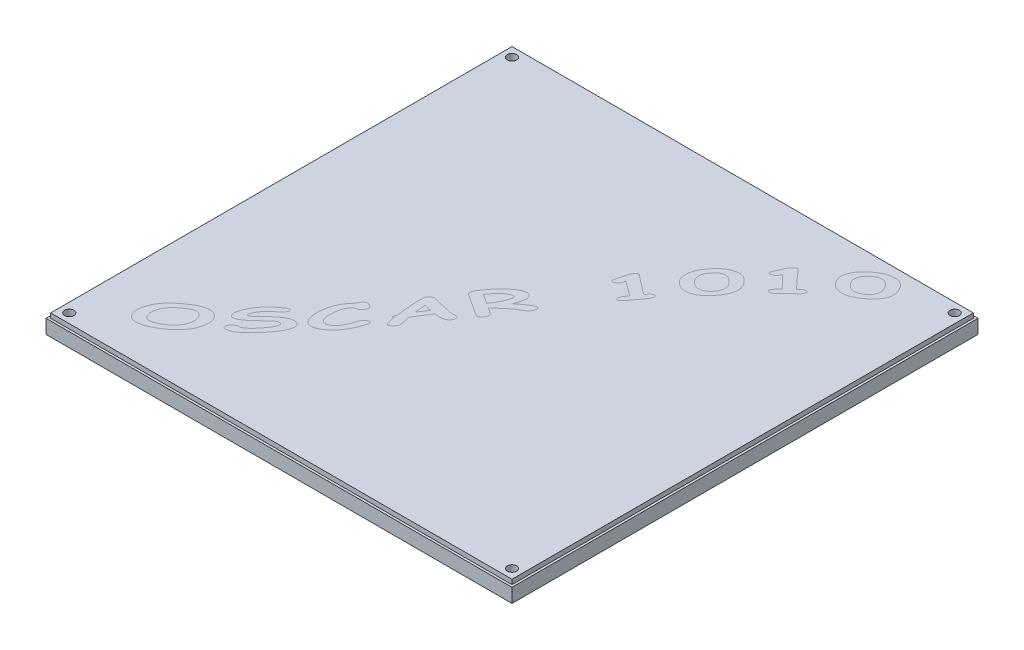
SolidWorks part; units mm, degrees
material "Brass"
ref_plane "Front Plane" through (0, 0, 0) normal (0, 0, 1) x (1, 0, 0)
ref_plane "Top Plane" through (0, 0, 0) normal (0, 1, 0) x (1, 0, 0)
ref_plane "Right Plane" through (0, 0, 0) normal (1, 0, 0) x (0, 0, -1)
sketch "Sketch1" plane through (0, 0, 0) normal (0, 1, 0) x (1, 0, 0)
  line L1 (100, -100) -> (-100, -100)
  line L2 (100, -100) -> (100, 100)
  line L3 (100, 100) -> (-100, 100)
  line L4 (-100, -100) -> (-100, 100)
  line L5 (100, -100) -> (-100, 100) construction
  line L6 (100, 100) -> (-100, -100) construction
  circle A0 centre (95, 95) radius 2
  circle A1 centre (95, -95) radius 2
  circle A2 centre (-95, -95) radius 2
  circle A3 centre (-95, 95) radius 2
  point P0 (0, 0)
  point P16 (0, 0)
  dimension "D3" = 4
  dimension "D4" = 95
  dimension "D1" = 200
  dimension "D2" = 200
  dimension "D5" = 4
extrude "Boss-Extrude1" add sketch "Sketch1" along normal blind 6
sketch "Sketch2" plane through (0, 6, 0) normal (0, 1, 0) x (1, 0, 0)
  line L1 (99, -99) -> (-99, -99)
  line L2 (99, -99) -> (99, 99)
  line L3 (99, 99) -> (-99, 99)
  line L4 (-99, -99) -> (-99, 99)
  line L5 (99, -99) -> (-99, 99) construction
  line L6 (99, 99) -> (-99, -99) construction
  point P0 (0, 0)
  dimension "D1" = 198
  dimension "D2" = 198
extrude "Boss-Extrude2" add sketch "Sketch2" along normal blind 2
sketch "Sketch3" plane through (0, 8, 0) normal (0, 1, 0) x (1, 0, 0)
  spline S0 degree 3 poles (-99, -99) (-0.1859, -51.0227) (0.1859, 51.0227) (99, 99) knots 0 0 0 0 1 1 1 1 construction
  text T0 "OSCAR 1010" font "Comic Sans MS" height in points 48
split line "Split Line3"
sketch "Sketch4" plane through (0, 8, 0) normal (0, 1, 0) x (1, 0, 0)
  circle A0 centre (-95, -95) radius 2 construction
  circle A1 centre (95, -95) radius 2 construction
  circle A2 centre (95, 95) radius 2 construction
  circle A3 centre (-95, 95) radius 2 construction
  circle A4 centre (-95, -95) radius 2
  circle A5 centre (95, -95) radius 2
  circle A6 centre (95, 95) radius 2
  circle A7 centre (-95, 95) radius 2
extrude "Cut-Extrude1" cut sketch "Sketch4" against normal through all
